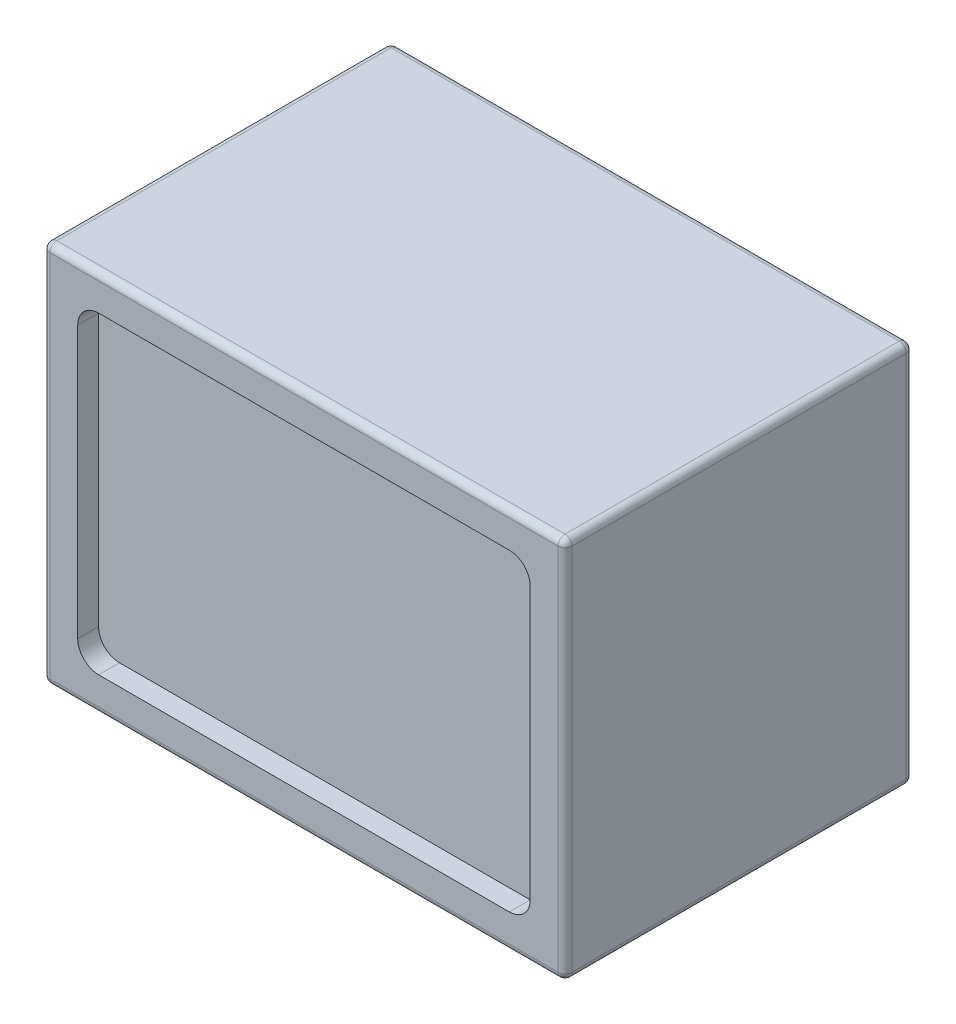
SolidWorks part; units mm, degrees
ref_plane "前视基准面" through (0, 0, 0) normal (0, 0, 1) x (1, 0, 0)
ref_plane "上视基准面" through (0, 0, 0) normal (0, 1, 0) x (1, 0, 0)
ref_plane "右视基准面" through (0, 0, 0) normal (1, 0, 0) x (0, 0, -1)
sketch "草图1" plane through (0, 0, 0) normal (0, 0, 1) x (1, 0, 0)
  line L1 (0, 0) -> (75, 0)
  line L2 (0, 0) -> (0, 55)
  line L3 (0, 55) -> (75, 55)
  line L4 (75, 0) -> (75, 55)
  dimension "D1" = 55
  dimension "D2" = 75
extrude "凸台-拉伸1" add sketch "草图1" along normal blind 50
sketch "草图2" plane through (0, 0, 50) normal (0, 0, 1) x (1, 0, 0)
  line L0 (0, 55) -> (0, 0) construction
  line L1 (5, 50) -> (70, 50)
  line L2 (5, 50) -> (5, 5)
  line L3 (5, 5) -> (70, 5)
  line L4 (70, 50) -> (70, 5)
  line L5 (75, 55) -> (0, 55) construction
  line L6 (75, 0) -> (75, 55) construction
  line L7 (0, 0) -> (75, 0) construction
  dimension "D1" = 5
  dimension "D2" = 5
  dimension "D3" = 5
  dimension "D4" = 5
extrude "切除-拉伸1" cut sketch "草图2" against normal blind 3
fillet "圆角1" radius 3 4 edges at (5, 5, 48.5) (70, 5, 48.5) (70, 50, 48.5) (5, 50, 48.5)
fillet "圆角2" radius 1 12 edges at (75, 27.5, 50) (75, 27.5, 0) (37.5, 0, 50) (75, 0, 25) (37.5, 0, 0) (75, 55, 25) (37.5, 55, 50) (37.5, 55, 0) (0, 55, 25) (0, 27.5, 50) (0, 0, 25) (0, 27.5, 0)
